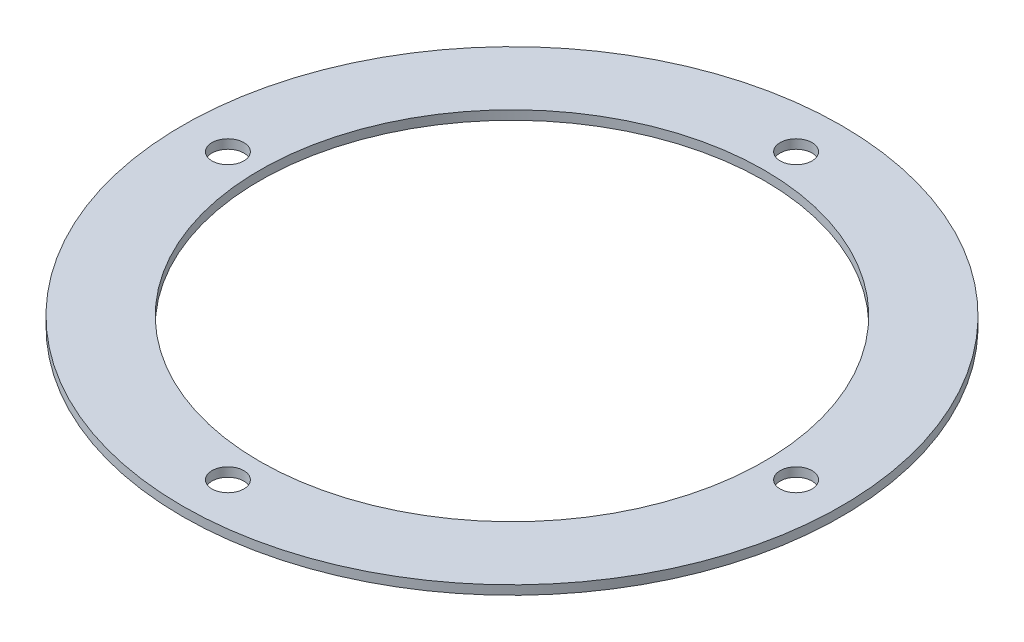
SolidWorks part; units mm, degrees
material "Q235-A"
ref_plane "Front Plane" through (0, 0, 0) normal (0, 0, 1) x (1, 0, 0)
ref_plane "Top Plane" through (0, 0, 0) normal (0, 1, 0) x (1, 0, 0)
ref_plane "Right Plane" through (0, 0, 0) normal (1, 0, 0) x (0, 0, -1)
sketch "Sketch1" plane through (0, 0, 0) normal (0, 1, 0) x (1, 0, 0)
  circle A0 centre (0, 0) radius 72.5
  circle A1 centre (0, 0) radius 55.5
  dimension "D1" = 145
  dimension "D2" = 111
extrude "Boss-Extrude1" add sketch "Sketch1" along normal blind 2
sketch "Sketch2" plane through (0, 2, 0) normal (0, 1, 0) x (1, 0, 0)
  circle A0 centre (0, 62.5) radius 3.5
  dimension "D1" = 7
  dimension "D2" = 62.5
extrude "Cut-Extrude1" cut sketch "Sketch2" against normal through all
pattern_circular "CirPattern1" count 4 over 360 about axis through (0, 0, 0) along (0, 1, 0) of "Cut-Extrude1"
